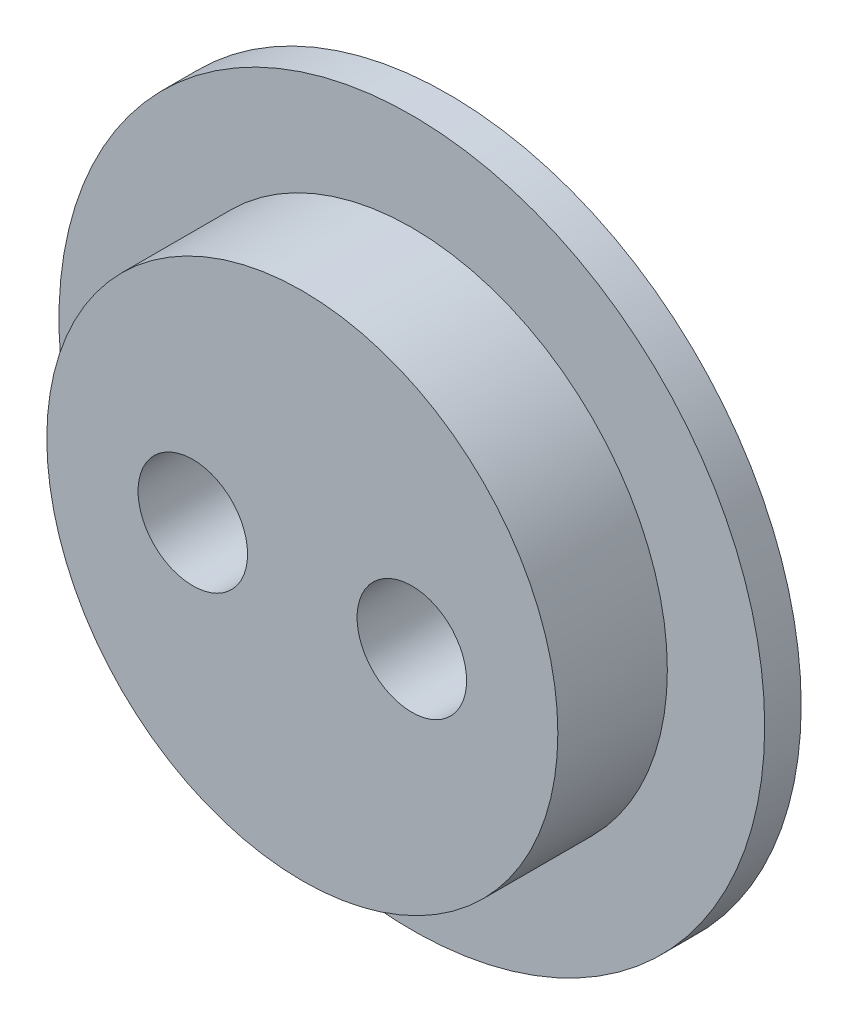
SolidWorks part; units mm, degrees
material "普通碳钢"
ref_plane "前视" through (0, 0, 0) normal (0, 0, 1) x (1, 0, 0)
ref_plane "上视" through (0, 0, 0) normal (0, 1, 0) x (1, 0, 0)
ref_plane "右视" through (0, 0, 0) normal (1, 0, 0) x (0, 0, -1)
sketch "草图1" plane through (0, 0, 0) normal (0, 0, 1) x (1, 0, 0)
  line L0 (-66.6844, 0) -> (59.6745, 0) construction
  line L1 (0, 52.5746) -> (0, -47.1824) construction
  circle A0 centre (0, 0) radius 29
  dimension "D1" = 58
extrude "凸台-拉伸1" add sketch "草图1" along normal blind 3
sketch "草图2" plane through (0, 0, 3) normal (0, 0, 1) x (1, 0, 0)
  circle A0 centre (0, 0) radius 21
  dimension "D1" = 42
extrude "凸台-拉伸2" add sketch "草图2" along normal blind 9
sketch "草图3" plane through (0, 0, 12) normal (0, 0, 1) x (1, 0, 0)
  line L0 (50, 0) -> (-50, 0) construction
  circle A0 centre (-9, 0) radius 4.5
  circle A1 centre (9, 0) radius 4.5
  dimension "D1" = 9
  dimension "D3" = 9
  dimension "D4" = 9
  dimension "D2" = 9
extrude "切除-拉伸1" cut sketch "草图3" against normal through all
